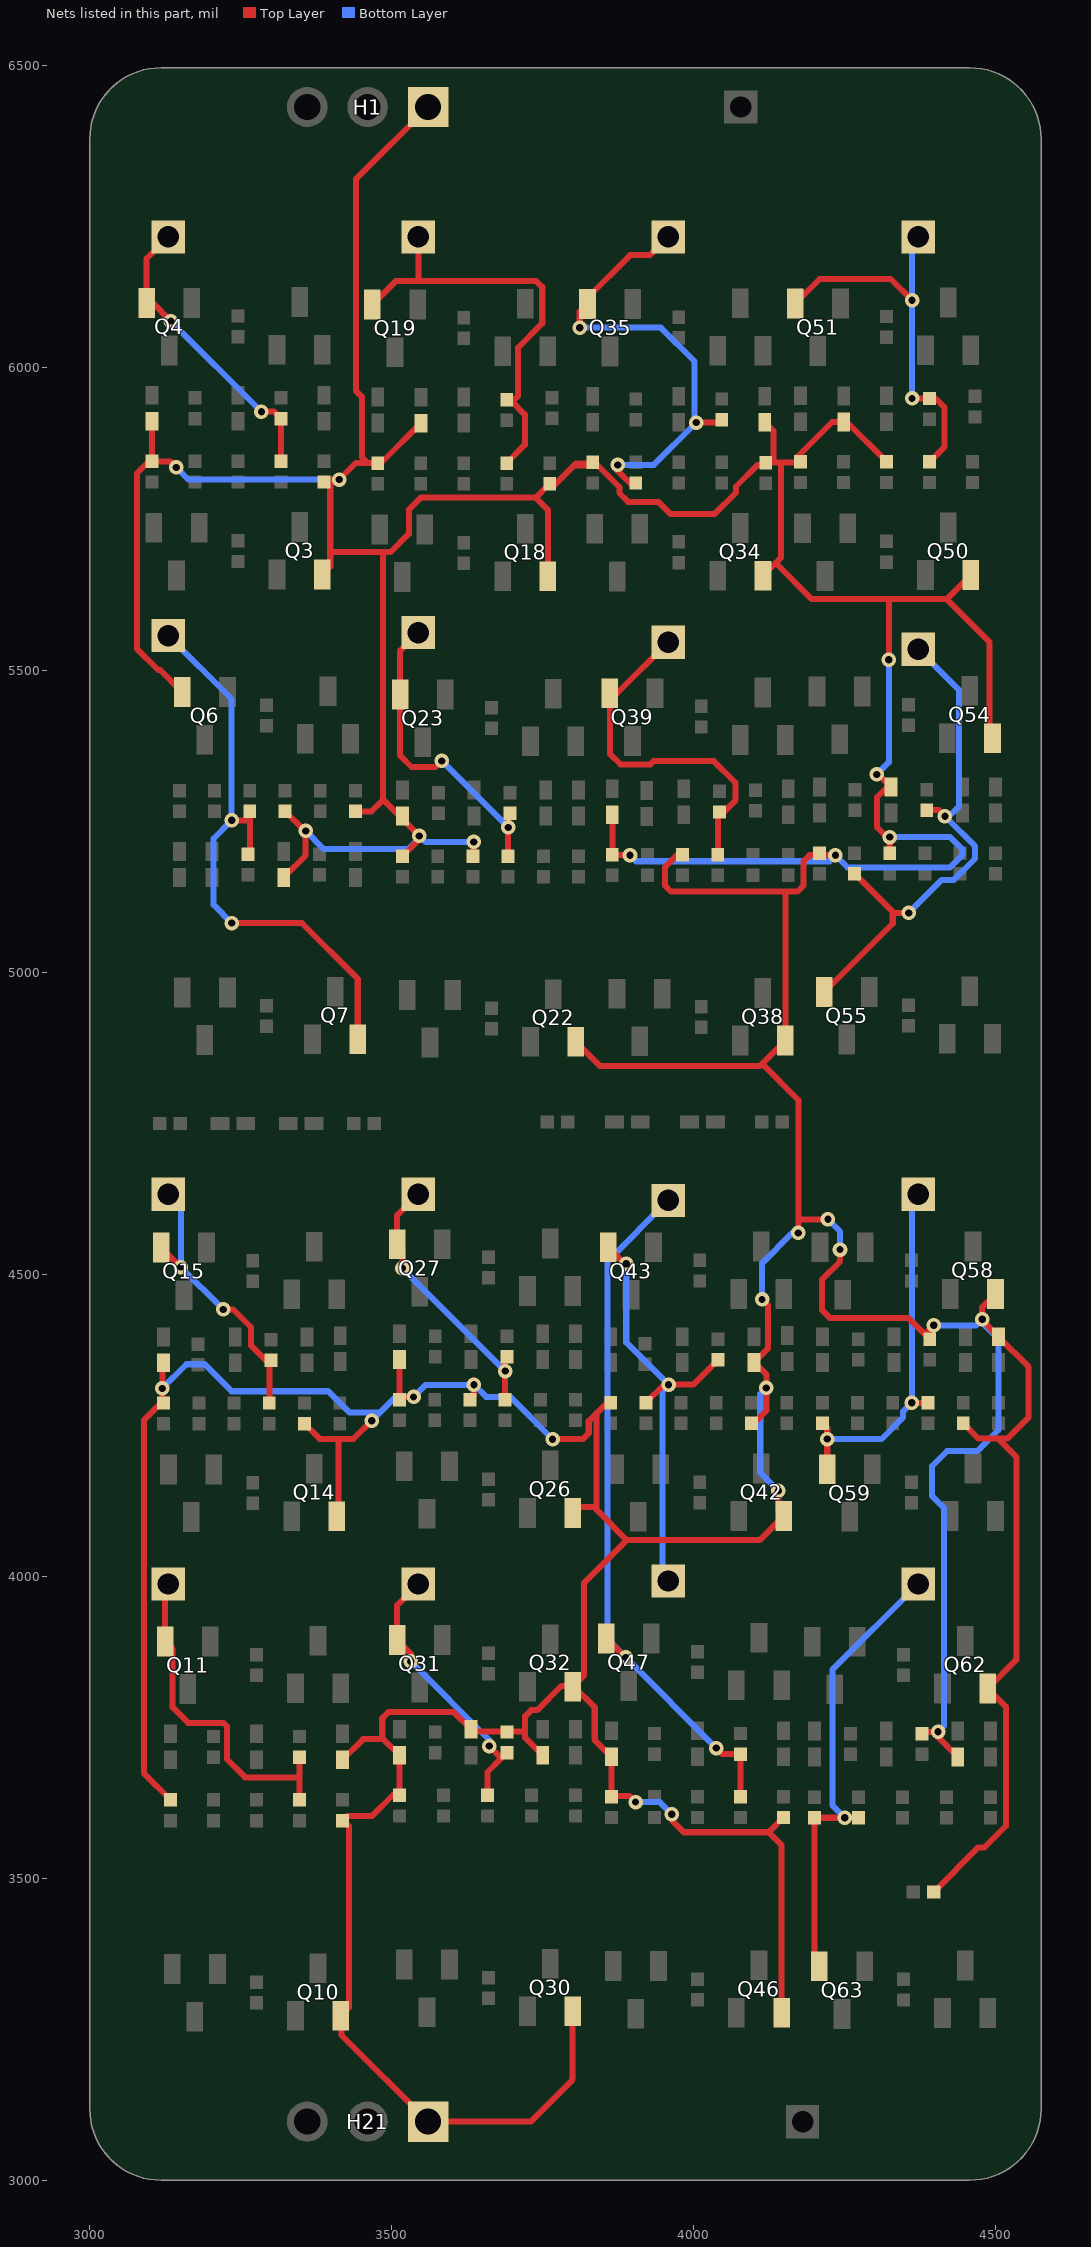
[diagram p0: the nets of this part, all layers, seen from the top]
# Altium PCB MISC61260.pcbdoc (part 4 of 4)
Units mil, origin at the board's own origin, x right, y up, seen from the top; angles counter-clockwise.
Board outline 1574.8 x 3497.01 mil, 2 copper layers (Top Layer, Bottom Layer), stack 62.206 mil thick; 303 components, 159 nets, 654 pads, 177 vias.

## Via types
v1: diameter 24.02, hole 12, Top Layer to Bottom Layer, 177 vias

## Nets (pads, with @x,y where several pads share a name; then routed paths per layer and width w, separated by ;. In a path a pad name is that pad's centre, name@x,y a point inside that pad or via, vN(x,y) a via of type N, cw(c..) or ccw(c..) an arc to the next point about the centre after c; other vN are vias at no path point) (continued)
V1: H6.1 Q19.2 Rp10.2 Rs10.1 | length 718.2
  Top Layer w10: Q19.2@3467.89,6105 3506.77,6143.88 3544.06,6143.88 ; H6.1@3543.75,6217.01 3544.06,6216.7 3544.06,6143.88 ; Rs10.1@3690.27,5842.67 3720.27,5872.67 3720.27,5922.67 Rp10.2@3699.06,5943.88 ; Rp10.2@3690.27,5947.67 3695.27,5947.67 Rp10.2@3699.06,5943.88 ; 3544.06,6143.88 3739.06,6143.88 3749.06,6133.88 3749.06,6073.88 3709.06,6033.88 3709.06,5953.88 Rp10.2@3699.06,5943.88
V1': H16.1 Q51.2 Rp26.2 Rs26.1 | length 657
  Top Layer w10: Q51.2@4167.89,6106.86 4208.41,6147.39 4325.89,6147.39 v1(4361.25,6112.03) ; v1(4361.25,5949.53) Rp26.2@4390.27,5949.53 4400.27,5949.53 4415.27,5934.53 4415.27,5869.53 Rs26.1@4390.27,5844.53
  Bottom Layer w10: v1(4361.25,5949.53) v1(4361.25,6112.03) 4361.25,6207.01 H16.1@4371.25,6217.01
V2: H7.1 Q23.2 Rp12.2 Rs12.1 | length 524.5
  Top Layer w10: H7.1@3543.75,5562.01 3513.9,5532.16 Q23.2@3513.9,5459.36 3513.9,5358.22 3532.59,5339.53 3572.59,5339.53 v1(3582.59,5349.53) ; Rs12.1@3692.59,5192.03 v1(3692.59,5239.53) 3692.59,5259.95 Rp12.2@3695.59,5262.95
  Bottom Layer w10: v1(3582.59,5349.53) v1(3692.59,5239.53)
V2': H17.1 Q55.2 Rp28.2 Rs28.1 | length 884.9
  Top Layer w10: Q55.2@4215.81,4967.01 4329.27,5080.47 4329.27,5099.72 ; Rs28.1@4266.03,5162.95 4329.27,5099.72 ; v1(4355.59,5097.95) 4331.03,5097.95 4329.27,5099.72 ; Rp28.2@4385.59,5267.95 4405.59,5267.95 v1(4415.59,5257.95)
  Bottom Layer w10: v1(4355.59,5097.95) 4410.24,5152.6 4430.24,5152.6 4465.59,5187.95 4465.59,5207.95 v1@4419.13,5254.42 ; H17.1@4371.25,5534.57 4439.13,5466.7 4439.13,5274.42 v1@4419.13,5254.42 ; v1(4415.59,5257.95) v1@4419.13,5254.42
V3: H9.1 Q27.2 Rp14.2 Rs14.1 | length 453.1
  Top Layer w10: v1(3517.59,4509.53) 3517.59,4540.67 Q27.2@3508.9,4549.36 3508.9,4597.16 H9.1@3543.75,4632.01 ; Rs14.1@3687.59,4292.03 v1(3687.59,4339.53) 3687.59,4359.95 Rp14.2@3690.59,4362.95
  Bottom Layer w10: v1(3517.59,4509.53) v1(3687.59,4339.53)
V3': H18.1 Q59.2 Rp30.2 Rs30.1 | length 626.1
  Top Layer w10: Rp30.2@4212.75,4252.95 4220.81,4244.89 v1(4220.81,4227.01) Q59.2@4220.81,4177.01 ; v1(4360.81,4287.01) Rs30.1@4387.59,4287.03
  Bottom Layer w10: v1(4220.81,4227.01) 4310.81,4227.01 4346.17,4262.37 4346.17,4272.37 v1(4360.81,4287.01) 4360.81,4621.57 H18.1@4371.25,4632.01
V4: H10.1 Q31.2 Rp16.2 Rs16.1 | length 458.3
  Top Layer w10: v1(3531.43,3858.79) 3531.43,3871.83 Q31.2@3508.9,3894.36 3508.9,3952.16 H10.1@3543.75,3987.01 ; Rs16.1@3658.45,3637.03 3658.45,3675.81 Rp16.2@3681.43,3698.79 ; v1(3661.43,3718.79) Rp16.2@3681.43,3698.79 ; Rp16.2@3690.59,3707.95 Rp16.2@3681.43,3698.79
  Bottom Layer w10: v1(3531.43,3858.79) 3661.43,3728.79 v1(3661.43,3718.79)
V4': H19.1 Q63.2 Rp32.2 Rs32.1 | length 776
  Top Layer w10: Q63.2@4207.89,3354.09 4199.83,3362.15 Rp32.2@4199.83,3600.03 v1(4249.83,3600.03) Rs32.1@4272.68,3600.03
  Bottom Layer w10: v1(4249.83,3600.03) 4229.83,3620.03 4229.83,3845.59 H19.1@4371.25,3987.01
V+: C4.1 C6.1 C10.1 C14.1 C18.1 C22.1 C26.1 C30.1 C31.1 C32.1 C33.1 C37.1 C41.1 C45.1 C49.1 C53.1 C57.1 C61.1 H1.1 H21.1 Q3.2 Q6.2 Q10.2 Q14.2 Q18.2 Q22.2 Q26.2 Q30.2 Q32.2 Q34.2 Q38.2 Q42.2 Q46.2 Q50.2 Q54.2 Q58.2 Q62.2 R4.1 R9.1 R13.1 R17.1 R20.1 R25.1 R29.1 R35.1 R39.1 R43.1 R47.1 R50.1 R55.1 R59.1 R63.1 Rp1.1 Rp3.1 Rp5.1 Rp7.1 Rp9.1 Rp11.1 Rp13.1 Rp15.1 Rp16.1 Rp17.1 Rp19.1 Rp21.1 Rp23.1 Rp25.1 Rp27.1 Rp29.1 Rp31.1 | length 16402.2
  Top Layer w10: C4.1@3103.12,5911.88 Rp1.1@3103.12,5845.38 ; Rp7.1@3122.33,4286.61 Rp7.1@3120.09,4288.85 ; C14.1@3122.33,4353.11 3120.09,4350.87 v1(3120.09,4310.76) Rp7.1@3120.09,4288.85 ; Rp5.1@3133.6,3629.53 3090.09,3673.04 3090.09,4258.85 Rp7.1@3120.09,4288.85 ; v1(3143.12,5835.38) 3133.12,5845.38 Rp1.1@3103.12,5845.38 ; Q6.2@3153.09,5463.52 3116.58,5500.03 3113.47,5500.03 3078.12,5535.38 3078.12,5825.38 3098.12,5845.38 Rp1.1@3103.12,5845.38 ; C6.1@3321.19,5156.72 3357.38,5192.92 v1(3357.38,5233.61) 3355.71,5233.61 R9.1@3323.19,5266.14 ; R17.1@3355.45,4252.53 3380.7,4227.28 3411.61,4227.28 ; Q3.2@3384.77,5658.01 3398.12,5671.35 3398.12,5695.38 ; R4.1@3387.83,5811.3 3391.91,5815.38 R4.1@3398.12,5815.38 ; Q14.2@3408.98,4099.23 3411.61,4101.86 3411.61,4227.28 ; Q10.2@3415.25,3272.15 Q10.2@3416.59,3273.49 ; R13.1@3418.31,3595.45 R13.1@3418.96,3596.1 ; C10.1@3418.31,3696.03 3452.61,3730.34 3485.95,3730.34 ; Rp3.1@3439.75,5266.14 3466.37,5266.14 3485.62,5285.38 ; v1(3466.61,4257.28) 3436.61,4227.28 3411.61,4227.28 ; Rp15.1@3512.75,3637.03 Rp15.1@3512.75,3638.53 ; C26.1@3512.75,4358.53 Rp13.1@3512.75,4292.03 3517.45,4296.73 v1(3536.05,4296.73) ; Rp11.1@3517.75,5192.03 3545.62,5219.89 v1(3545.62,5225.38) C22.1@3517.44,5253.56 ; C22.1@3517.75,5258.53 C22.1@3517.44,5253.56 ; C18.1@3548.14,5908.69 3482.12,5842.67 Rp9.1@3476.74,5842.67 3460.4,5842.67 ; H1.1@3560,6432.01 3440.4,6312.41 3440.4,5962.67 3450.4,5952.67 3450.4,5852.67 3460.4,5842.67 ; R29.1@3629.31,4292.03 3636.05,4298.77 v1(3636.05,4316.73) ; R25.1@3634.31,5192.03 3635.62,5193.33 v1(3635.62,5215.38) ; Rp16.1@3690.59,3742.03 Rp16.1@3691.75,3743.19 ; C32.1@3749.87,3703.53 3720.59,3732.81 3720.59,3743.19 ; Q18.2@3758.39,5655.29 3758.39,5765.23 3738.24,5785.38 ; R20.1@3761.45,5808.59 R20.1@3759.45,5806.6 ; v1(3766.05,4226.73) 3816.05,4226.73 3826.05,4236.73 3826.05,4256.73 3838.98,4269.65 ; Q30.2@3799.41,3279.65 3799.41,3166.41 3730,3097.01 H21.1@3560,3097.01 3416.59,3240.42 Q10.2@3416.59,3273.49 ; Q32.2@3799.41,3817 Q32.2@3800.59,3818.19 ; Q26.2@3799.41,4104.65 3809.41,4114.65 3838.98,4114.65 ; Q22.2@3804.41,4884.65 3844.41,4844.65 4109.41,4844.65 4112.92,4848.17 ; Rp17.1@3832.75,5843.69 3831.02,5841.95 3804.81,5841.95 3801.27,5838.42 ; Rp21.1@3862.33,4287.03 3856.36,4287.03 3838.98,4269.65 ; Rp23.1@3863.6,3634.53 Rp23.1@3863.6,3636.03 ; Rp19.1@3864.83,5194.11 Rp19.1@3865.49,5193.45 ; C37.1@3864.83,5260.61 3865.49,5259.95 Rp19.1@3865.49,5193.45 ; v1(3894.31,5193.45) Rp19.1@3865.49,5193.45 ; v1(3903.6,3626.03) 3893.6,3636.03 Rp23.1@3863.6,3636.03 ; v1(3963.6,3606.03) 3963.6,3596.03 3983.6,3576.03 4123.89,3576.03 ; R39.1@3981.39,5194.11 3972.7,5194.11 3952.05,5173.45 3952.05,5143.45 3962.05,5133.45 4151.81,5133.45 ; R43.1@4095.45,4252.95 4098.87,4252.95 4119.94,4274.02 v1(4119.94,4311.52) 4119.94,4334.02 C41.1@4099.94,4354.02 ; C41.1@4099.45,4353.53 C41.1@4099.94,4354.02 ; v1(4112.92,4458.17) 4122.92,4448.17 4122.92,4377 C41.1@4099.94,4354.02 ; Q34.2@4114.41,5656.31 4135.32,5677.22 ; C33.1@4117.46,5910.19 4131.65,5895.99 4131.65,5843.2 ; v1(4139.94,4141.52) 4139.94,4108.7 Q42.2@4148.98,4099.65 4108.98,4059.65 3888.98,4059.65 ; Q46.2@4145.25,3277.15 4145.25,3554.67 4123.89,3576.03 ; R47.1@4148.31,3600.45 4123.89,3576.03 ; v1(4172.92,4568.17) 4172.92,4590.67 ; Rp25.1@4176.74,5844.53 4175.41,5843.2 Rp25.1@4171.65,5843.2 ; Rp27.1@4207.75,5197.03 Rp27.1@4211.33,5193.45 ; v1(4221.95,4590.67) 4172.92,4590.67 ; v1(4234.31,5193.45) Rp27.1@4211.33,5193.45 ; v1(4241.95,4540.67) 4241.95,4520.67 4211.95,4490.67 4211.95,4440.67 4224.95,4427.68 4354.95,4427.68 Rp29.1@4387.31,4395.32 ; v1(4302.82,5327.22) 4305.55,5327.22 C53.1@4323.22,5309.54 ; R50.1@4319.09,5844.53 4253.07,5910.55 C49.1@4248.14,5910.55 4229,5910.55 4171.65,5853.2 Rp25.1@4171.65,5843.2 ; v1(4322.82,5517.22) 4322.82,5617.22 ; R55.1@4324.31,5197.03 v1@4324.31,5218.45 ; v1(4324.31,5223.45) v1@4324.31,5218.45 ; C53.1@4326.31,5306.45 C53.1@4323.22,5309.54 ; Rp31.1@4377.67,3739.11 4380.95,3742.39 v1(4404.38,3742.39) 4404.38,3733.18 C61.1@4436.95,3700.61 ; Rp29.1@4390.59,4392.03 Rp29.1@4387.31,4395.32 ; R63.1@4397.04,3477.01 4471.13,3551.09 4481.13,3551.09 4516.48,3586.45 4516.48,3784.08 Q62.2@4486.48,3814.08 4533.8,3861.39 4533.8,4197.6 4503.8,4227.6 ; v1(4397.31,4415.32) 4387.31,4405.32 Rp29.1@4387.31,4395.32 ; R59.1@4445.87,4252.95 4471.23,4227.6 4503.8,4227.6 ; Q50.2@4458.39,5657.15 4418.45,5617.22 ; Q54.2@4494.41,5387 4489.16,5392.24 4489.16,5546.51 4418.45,5617.22 ; Q58.2@4499.41,4467 4477.31,4444.9 v1(4477.31,4425.32) 4477.31,4423.3 C57.1@4504.15,4396.45 4554.15,4346.45 4554.15,4262.95 4518.8,4227.6 4503.8,4227.6 ; 3398.12,5695.38 R4.1@3398.12,5815.38 ; 3398.12,5695.38 3485.62,5695.38 ; R4.1@3398.12,5815.38 v1(3413.12,5815.38) 3440.4,5842.67 3460.4,5842.67 ; Q10.2@3416.59,3273.49 3428.96,3285.87 3428.96,3586.1 R13.1@3418.96,3596.1 ; R13.1@3418.96,3596.1 3426.03,3603.18 3467.4,3603.18 3502.75,3638.53 Rp15.1@3512.75,3638.53 ; 3485.62,5285.38 3485.62,5695.38 ; 3485.62,5285.38 C22.1@3517.44,5253.56 ; 3485.62,5695.38 3498.12,5695.38 3528.12,5725.38 3528.12,5765.38 3548.12,5785.38 3738.24,5785.38 ; 3485.95,3730.34 3484.18,3732.1 3484.18,3764.96 3494.18,3774.96 3602.81,3774.96 C31.1@3631.31,3746.45 3634.57,3743.19 Rp16.1@3691.75,3743.19 ; 3485.95,3730.34 C30.1@3512.75,3703.53 Rp15.1@3512.75,3638.53 ; Rp16.1@3691.75,3743.19 3720.59,3743.19 ; 3720.59,3743.19 3720.59,3768.19 3730.59,3778.19 3740.59,3778.19 3780.59,3818.19 Q32.2@3800.59,3818.19 ; 3738.24,5785.38 R20.1@3759.45,5806.6 ; R20.1@3759.45,5806.6 3769.45,5806.6 3801.27,5838.42 ; Q32.2@3800.59,3818.19 3835.95,3782.83 3835.95,3728.68 C45.1@3863.6,3701.03 Rp23.1@3863.6,3636.03 ; Q32.2@3800.59,3818.19 3818.27,3835.87 3818.27,3988.94 3888.98,4059.65 ; 3801.27,5838.42 3841.27,5838.42 3876.63,5803.06 3876.63,5793.06 3891.27,5778.42 3941.27,5778.42 3961.27,5758.42 4034.37,5758.42 4069.72,5793.77 4069.72,5803.77 4105.08,5839.13 4115.08,5839.13 R35.1@4119.15,5843.2 4131.65,5843.2 ; 3838.98,4114.65 3838.98,4109.65 3888.98,4059.65 ; 3838.98,4114.65 3838.98,4269.65 ; 4112.92,4848.17 4172.92,4788.17 4172.92,4590.67 ; 4112.92,4848.17 4151.81,4887.06 4151.81,5133.45 ; 4131.65,5843.2 4144.15,5843.2 ; 4135.32,5677.22 4195.32,5617.22 4322.82,5617.22 ; 4135.32,5677.22 4144.15,5686.06 4144.15,5843.2 ; 4144.15,5843.2 Rp25.1@4171.65,5843.2 ; 4151.81,5133.45 4171.81,5133.45 4181.81,5143.45 4181.81,5183.45 4191.81,5193.45 Rp27.1@4211.33,5193.45 ; 4322.82,5617.22 4418.45,5617.22 ; C53.1@4323.22,5309.54 4303.22,5289.54 4303.22,5239.54 v1@4324.31,5218.45
  Bottom Layer w10: v1(3120.09,4310.76) 3160.09,4350.76 3190.09,4350.76 3234.74,4306.12 3394.74,4306.12 3430.09,4270.76 3480.09,4270.76 ; v1(3143.12,5835.38) 3163.12,5815.38 v1(3413.12,5815.38) ; v1(3357.38,5233.61) 3387.38,5203.61 3527.38,5203.61 v1@3547.38,5223.61 ; v1(3466.61,4257.28) 3480.09,4270.76 ; v1(3536.05,4296.73) v1@3536.61,4297.28 ; v1(3545.62,5225.38) v1@3547.38,5223.61 ; v1(3635.62,5215.38) 3555.62,5215.38 v1@3547.38,5223.61 ; v1(3766.05,4226.73) 3696.05,4296.73 3656.05,4296.73 v1(3636.05,4316.73) 3556.05,4316.73 v1@3536.61,4297.28 ; v1(3894.31,5193.45) 3904.31,5183.45 4224.31,5183.45 v1(4234.31,5193.45) 4254.31,5173.45 4424.31,5173.45 4444.31,5193.45 4444.31,5203.45 4424.31,5223.45 v1(4324.31,5223.45) ; v1(3903.6,3626.03) 3943.6,3626.03 v1(3963.6,3606.03) ; v1(4112.92,4458.17) 4112.92,4518.17 4162.92,4568.17 v1(4172.92,4568.17) ; v1(4119.94,4311.52) 4109.94,4301.52 4109.94,4171.52 v1(4139.94,4141.52) ; v1(4221.95,4590.67) 4241.95,4570.67 v1(4241.95,4540.67) ; v1(4302.82,5327.22) 4322.82,5347.22 v1(4322.82,5517.22) ; v1(4397.31,4415.32) 4467.31,4415.32 v1@4474.38,4422.39 ; v1(4404.38,3742.39) 4414.38,3752.39 4414.38,4112.39 4394.38,4132.39 4394.38,4182.39 4419.02,4207.03 4469.02,4207.03 4504.38,4242.39 4504.38,4392.39 v1@4474.38,4422.39 ; v1(4477.31,4425.32) v1@4474.38,4422.39 ; 3480.09,4270.76 3506.61,4297.28 v1@3536.61,4297.28
VL1: H2.1 Q4.2 Rp2.2 Rs2.1 | length 496.7
  Top Layer w10: H2.1@3130,6217.01 3094.27,6181.27 Q4.2@3094.27,6107.71 3104.27,6107.71 v1(3134.27,6077.71) ; v1(3284.27,5927.71) 3305.24,5927.71 Rp2.2@3316.65,5916.3 Rs2.1@3316.65,5845.38
  Bottom Layer w10: v1(3134.27,6077.71) v1(3284.27,5927.71)
VL1': H12.1 Q35.2 Rp18.2 Rs18.1 | length 798.9
  Top Layer w10: v1(3811.11,6066.78) 3811.11,6093.22 Q35.2@3823.9,6106.02 3823.9,6116.02 3894.61,6186.73 3927.22,6186.73 H12.1@3957.5,6217.01 ; v1(3873.93,5839.6) 3873.93,5829.6 3893.93,5809.6 Rs18.1@3903.93,5809.6 ; v1(4003.93,5909.6) 4041.29,5909.6 Rp18.2@4046.29,5914.6
  Bottom Layer w10: v1(3811.11,6066.78) 3945.23,6066.78 4001.11,6010.9 v1@4001.11,5906.78 ; v1(3873.93,5839.6) 3933.93,5839.6 v1@4001.11,5906.78 ; v1(4003.93,5909.6) v1@4001.11,5906.78
VL2: H3.1 Q7.2 Rp4.2 Rs4.1 | length 993.3
  Top Layer w10: v1(3234.91,5081.14) 3351.27,5081.14 3443.6,4988.81 Q7.2@3443.6,4888.81 ; v1(3234.91,5251.14) 3264.91,5251.14 ; Rp4.2@3261.91,5195.22 3264.91,5198.22 3264.91,5251.14 ; Rs4.1@3264.91,5266.14 3264.91,5251.14
  Bottom Layer w10: H3.1@3130,5557.01 3234.91,5452.1 v1(3234.91,5251.14) 3204.91,5221.14 3204.91,5111.14 v1(3234.91,5081.14)
VL2': H13.1 Q39.2 Rp20.2 Rs20.1 | length 601.1
  Top Layer w10: H13.1@3957.5,5546.15 3872.79,5461.44 Q39.2@3860.98,5461.44 3860.98,5361.44 3878.62,5343.8 3927.91,5343.8 3933.27,5349.15 4033.27,5349.15 4068.62,5313.8 4068.62,5283.8 4048.62,5263.8 Rp20.2@4041.44,5263.8 ; Rs20.1@4039.67,5194.11 4039.67,5262.03 Rp20.2@4041.44,5263.8 ; Rp20.2@4042.67,5265.03 Rp20.2@4041.44,5263.8
VR1: H5.1 Q11.2 Rp6.2 Rs6.1 | length 572.2
  Top Layer w10: H5.1@3130,3987.01 3124.75,3981.76 Q11.2@3124.75,3891.86 3137.13,3879.48 3137.13,3782.8 3162.9,3757.03 3221.37,3757.03 3227.13,3751.27 3227.13,3697.03 3257.13,3667.03 3347.13,3667.03 ; Rs6.1@3347.13,3629.53 3347.13,3667.03 ; Rp6.2@3347.13,3700.45 3347.13,3667.03
VR1': H15.1 Q43.2 Rp22.2 Rs22.1 | length 751.9
  Top Layer w10: Q43.2@3858.48,4544.36 3885.81,4517.03 v1(3888.11,4517.03) ; Rs22.1@3920.61,4287.03 3950.61,4317.03 3999.25,4317.03 Rp22.2@4040.17,4357.95
  Bottom Layer w10: v1(3888.11,4517.03) 3888.11,4387.03 v1(3958.11,4317.03) 3948.11,4307.03 3948.11,4001.4 H15.1@3957.5,3992.01
VR2: H4.1 Q15.2 Rp8.2 Rs8.1 | length 477.1
  Top Layer w10: Q15.2@3118.48,4543.94 v1(3150.81,4511.61) ; v1(3220.81,4441.61) 3237.17,4441.61 3267.17,4411.61 3267.17,4381.61 Rp8.2@3297.17,4351.61 ; Rs8.1@3297.17,4286.61 Rp8.2@3297.17,4351.61 ; Rp8.2@3300.17,4357.53 3297.17,4354.53 Rp8.2@3297.17,4351.61
  Bottom Layer w10: H4.1@3130,4632.01 3150.81,4611.2 v1(3150.81,4511.61) v1(3220.81,4441.61)
VR2': H14.1 Q47.2 Rp24.2 Rs24.1 | length 1183.1
  Top Layer w10: Q47.2@3854.75,3896.86 3886.16,3865.45 v1(3887.13,3865.45) ; v1(4037.13,3715.45) 4047.13,3705.45 Rp24.2@4077.13,3705.45 Rs24.1@4077.13,3634.53
  Bottom Layer w10: H14.1@3957.5,4622.01 3857.13,4521.64 3857.13,3895.45 v1(3887.13,3865.45) v1(4037.13,3715.45)

## Keep-outs
Board Outline Layer:
  the board outline again, w10

## Other copper
Top Layer:
  drawing of 989 lines, arcs and shapes, not listed
Bottom Layer:
  drawing of 208 lines, arcs and shapes, not listed

## Silkscreen, mask and mechanical layers (free items; w line width, h text height)
Bottom Silkscreen Layer:
  text "GND" at 3390,6312.01 h78.74
  text "B1" at 3505,6312.01 h78.74
  text "V+" at 3670,6312.01 h78.74
  text "B2" at 4115,6312.01 h78.74
  text "VL1" at 3189.1,6092.01 h78.74
  text "V1" at 3580.3,6092.01 h78.74
  text "VL1'" at 4028.1,6087.01 h78.74
  text "V1'" at 4425,6087.01 h78.74
  text "VL2" at 3199.05,5427.01 h78.74
  text "V2" at 3590.25,5425.91 h78.74
  text "VL2'" at 4038.05,5409.7 h78.74
  text "V2'" at 4429.25,5400.37 h78.74
  text "VR2" at 3201.3,4497.01 h78.74
  text "V3" at 3590.25,4497.01 h78.74
  text "V3'" at 4429.25,4497.01 h78.74
  text "VR2'" at 4040.3,4487.01 h78.74
  text "VR1'" at 4030.35,3857.01 h78.74
  text "VR1" at 3191.35,3852.01 h78.74
  text "V4" at 3591.35,3852.01 h78.74
  text "V4'" at 4430.35,3852.01 h78.74
  text "GND" at 3405,3152.01 h78.74
  text "B1" at 3495,3152.01 h78.74
  text "V+" at 3645,3152.01 h78.74
  text "B2'" at 4230,3142.01 h78.74